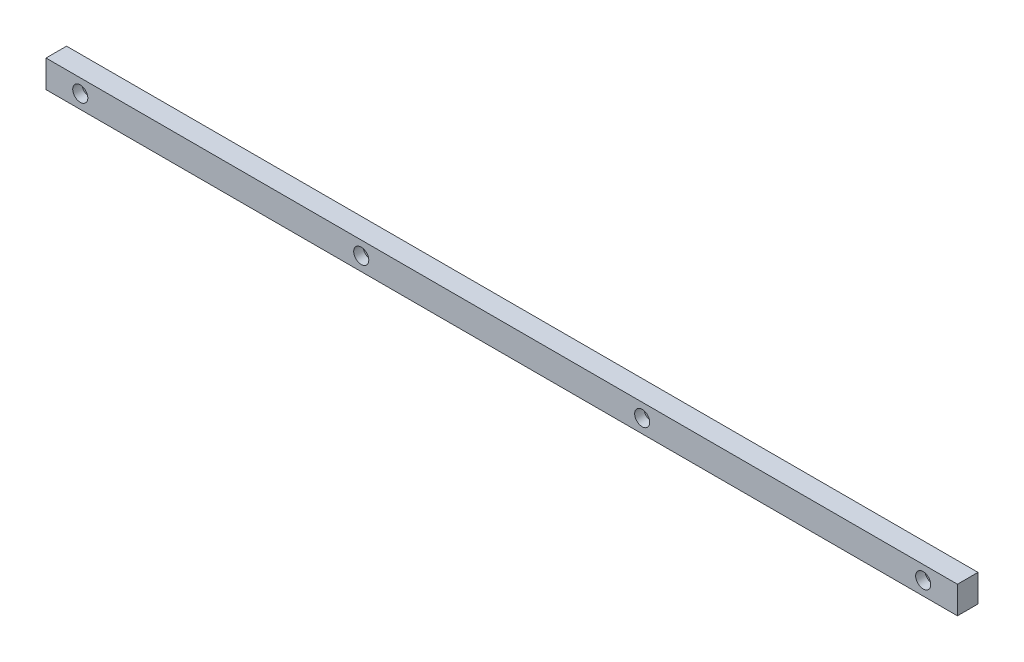
from build123d import *

# Parameters (mm, degrees)
SKETCH_1_W                = 665
SKETCH_1_H                = 20
EXTRUDE_1_DEPTH           = 15
HOLE_WIZARD_1_D           = 6.6
HOLE_WIZARD_1_CBORE_D     = 11
HOLE_WIZARD_1_CBORE_DEPTH = 6.8


with BuildPart() as part:
    # 草图1 → 凸台-拉伸1 (new body)
    with BuildSketch(Plane.XY):
        Rectangle(SKETCH_1_W, SKETCH_1_H)
    extrude(amount=EXTRUDE_1_DEPTH)

    # 打孔尺寸(%根据)内六角圆柱头螺钉的类型1 (through all)
    with Locations(Plane.XY.offset(15)):
        with Locations((102.5, 0), (-307.5, 0), (307.5, 0), (-102.5, 0)):
            CounterBoreHole(HOLE_WIZARD_1_D / 2, HOLE_WIZARD_1_CBORE_D / 2, HOLE_WIZARD_1_CBORE_DEPTH)


solid = part.part
